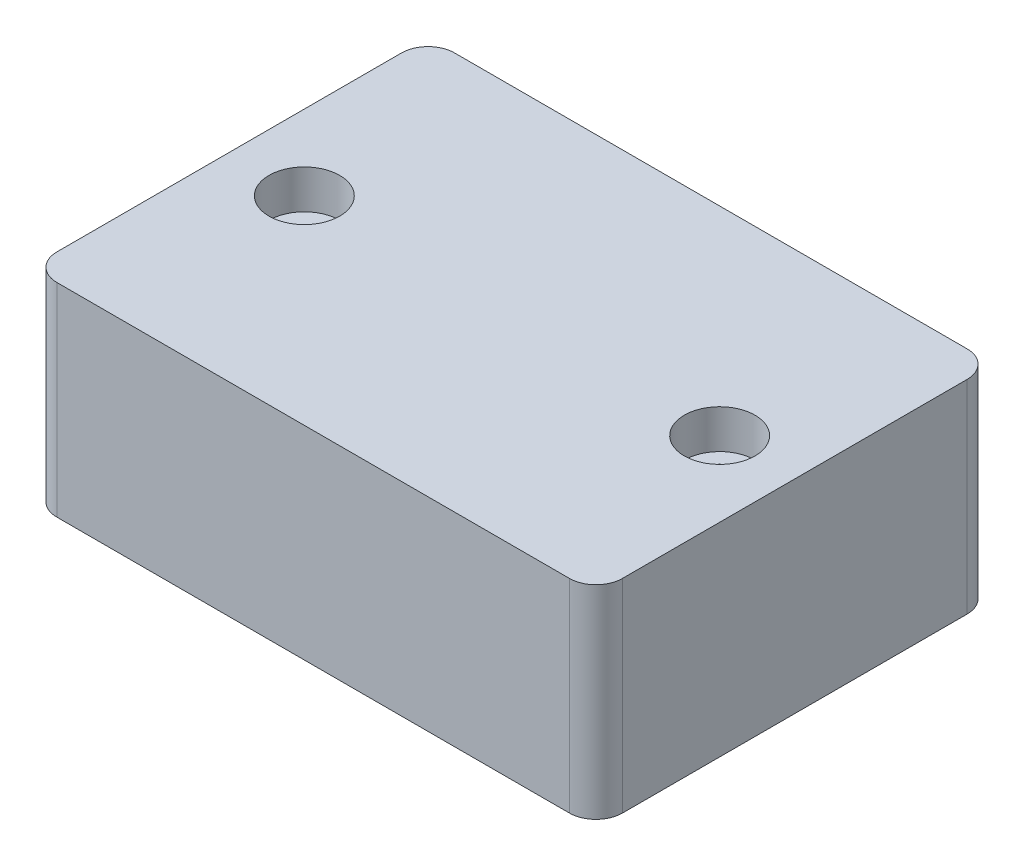
SolidWorks part; units mm, degrees
material "标准件"
ref_plane "前视基准面" through (0, 0, 0) normal (0, 0, 1) x (1, 0, 0)
ref_plane "上视基准面" through (0, 0, 0) normal (0, 1, 0) x (1, 0, 0)
ref_plane "右视基准面" through (0, 0, 0) normal (1, 0, 0) x (0, 0, -1)
sketch "草图1" plane through (0, 0, 0) normal (0, 1, 0) x (1, 0, 0)
  line L1 (-32, -22.5) -> (32, -22.5)
  line L2 (-32, -22.5) -> (-32, 22.5)
  line L3 (-32, 22.5) -> (32, 22.5)
  line L4 (32, -22.5) -> (32, 22.5)
  line L5 (-32, -22.5) -> (32, 22.5) construction
  line L6 (-32, 22.5) -> (32, -22.5) construction
  point P0 (0, 0)
  dimension "D1" = 64
  dimension "D2" = 45
extrude "凸台-拉伸1" add sketch "草图1" along normal mid plane 23
hole_wizard "M4 六角凹头螺钉的柱形沉头孔1" positions "草图2" profile "草图3" counterbore size "M4" standard "ISO" end condition through all
sketch "草图2" plane through (0, 11.5, 0) normal (0, 1, 0) x (1, 0, 0)
  line L0 (0, 0) -> (0, 32.2434) construction
  point P0 (-23.5, 0)
  point P2 (23.5, 0)
  dimension "D1" = 47
sketch "草图3" plane through (-23.5, 11.5, 0) normal (1, 0, 0) x (0, 0, 1)
  line L0 (0, 0) -> (0, 23)
  line L1 (0, 23) -> (2.25, 23)
  line L3 (2.25, 23) -> (2.25, 4.4)
  line L4 (2.25, 4.4) -> (4, 4.4)
  line L5 (4, 4.4) -> (4, 0)
  line L7 (4, 0) -> (0, 0)
  line L11 (0, -6.35) -> (0, 107.95) construction
  dimension "通孔孔直径" = 4.5
  dimension "通孔孔深度" = 23
  dimension "柱形沉头孔直径" = 8
  dimension "柱形沉头孔深度" = 4.4
fillet "圆角1" radius 3 4 edges at (32, 0, 22.5) (32, 0, -22.5) (-32, 0, -22.5) (-32, 0, 22.5)
